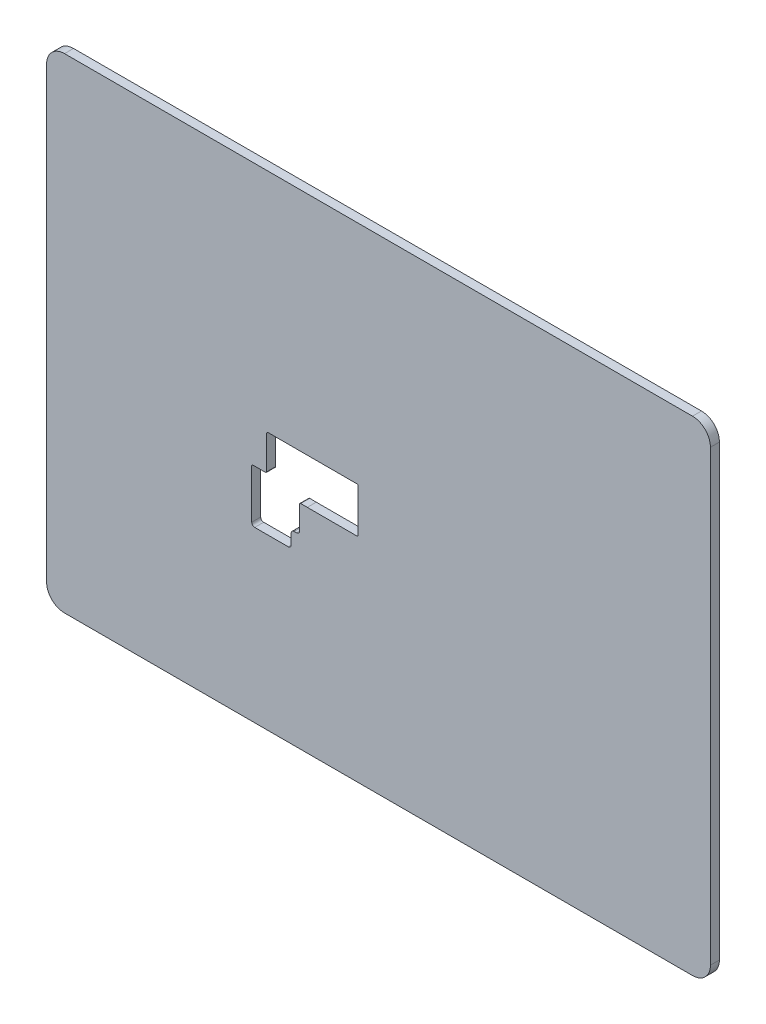
SolidWorks part; units mm, degrees
ref_plane "前视基准面" through (0, 0, 0) normal (0, 0, 1) x (1, 0, 0)
ref_plane "上视基准面" through (0, 0, 0) normal (0, 1, 0) x (1, 0, 0)
ref_plane "右视基准面" through (0, 0, 0) normal (1, 0, 0) x (0, 0, -1)
sketch "草图1" plane through (0, 0, 0) normal (0, 0, 1) x (1, 0, 0)
  line L2 (-456.7544, 478.7406) -> (-456.7544, -271.2594)
  line L5 (-426.7544, 508.7406) -> (623.2456, 508.7406)
  line L6 (653.2456, 478.7406) -> (653.2456, -271.2594)
  line L7 (623.2456, -301.2594) -> (-426.7544, -301.2594)
  arc A4 (-426.7544, 508.7406) -> (-456.7544, 478.7406) centre (-426.7544, 478.7406) ccw
  arc A5 (-456.7544, -271.2594) -> (-426.7544, -301.2594) centre (-426.7544, -271.2594) ccw
  arc A6 (623.2456, -301.2594) -> (653.2456, -271.2594) centre (623.2456, -271.2594) ccw
  arc A7 (653.2456, 478.7406) -> (623.2456, 508.7406) centre (623.2456, 478.7406) ccw
  dimension "D2" = 30
  dimension "D4" = 30
  dimension "D6" = 30
  dimension "D7" = 30
  dimension "D9" = 1050
  dimension "D10" = 750
extrude "凸台-拉伸1" add sketch "草图1" along normal blind 15
sketch "草图2" plane through (0, 0, 15) normal (0, 0, 1) x (1, 0, 0)
  line L8 (-113.7544, 51.6781) -> (-113.7544, -13.3219)
  line L9 (-108.7544, -18.3219) -> (-52.7544, -18.3219)
  line L10 (-426.7544, -301.2594) -> (623.2456, -301.2594)
  line L11 (-426.7544, -301.2594) -> (-456.7544, -301.2594)
  line L13 (-47.7544, -13.3219) -> (-47.7544, 3.7468)
  line L18 (-113.7544, 68.4296) -> (-113.7544, 51.6781)
  line L22 (-20.8646, 54.6761) -> (-31.7553, 54.7343)
  line L25 (-42.8236, 8.7464) -> (-38.6852, 8.8036)
  line L27 (-33.7544, 51.6781) -> (-33.7544, 13.8031)
  line L28 (-33.7544, 51.6781) -> (-33.7544, 53.2415)
  line L46 (-88.6922, 100.216) -> (-88.6922, 128.216)
  line L47 (-88.6922, 100.216) -> (-88.6922, 72.4296)
  line L48 (-90.6922, 70.4296) -> (-111.7544, 70.4296)
  line L53 (-86.6922, 130.216) -> (62.1971, 130.216)
  line L54 (64.1971, 89.9756) -> (64.1971, 56.6761)
  line L55 (-20.8646, 54.6761) -> (62.1971, 54.6761)
  line L56 (64.1971, 128.216) -> (64.1971, 89.9756)
  arc A12 (-52.7544, -18.3219) -> (-47.7544, -13.3219) centre (-52.7544, -13.3219) ccw
  arc A13 (-108.7544, -18.3219) -> (-113.7544, -13.3219) centre (-108.7544, -13.3219) cw
  arc A15 (-33.7544, 53.2415) -> (-31.7553, 54.7343) centre (-31.8195, 52.7353) cw
  arc A16 (-33.7544, 13.8031) -> (-38.6852, 8.8036) centre (-38.7544, 13.8031) cw
  arc A17 (-47.7544, 3.7468) -> (-42.8236, 8.7464) centre (-42.7544, 3.7468) cw
  arc A34 (62.1971, 54.6761) -> (64.1971, 56.6761) centre (62.1971, 56.6761) ccw
  arc A36 (-113.7544, 68.4296) -> (-111.7544, 70.4296) centre (-111.7544, 68.4296) cw
  arc A37 (-90.6922, 70.4296) -> (-88.6922, 72.4296) centre (-90.6922, 72.4296) ccw
  arc A39 (62.1971, 130.216) -> (64.1971, 128.216) centre (62.1971, 128.216) cw
  arc A40 (-86.6922, 130.216) -> (-88.6922, 128.216) centre (-86.6922, 128.216) ccw
  point P21 (-47.7544, 8.7406)
  point P27 (-88.6922, 130.216)
  point P30 (57.5727, 54.8271)
  point P46 (-113.7544, -18.2594)
  dimension "D1" = 2
  dimension "D2" = 30
  dimension "D3" = 2
extrude "切除-拉伸1" cut sketch "草图2" against normal through all contours L22 A15 L28 L27 A16 L25 A17 L13 A12 L9 A13 L8 L18 A36 L48 A37 L47 L46 A40 L53 A39 L56 L54 A34 L55
